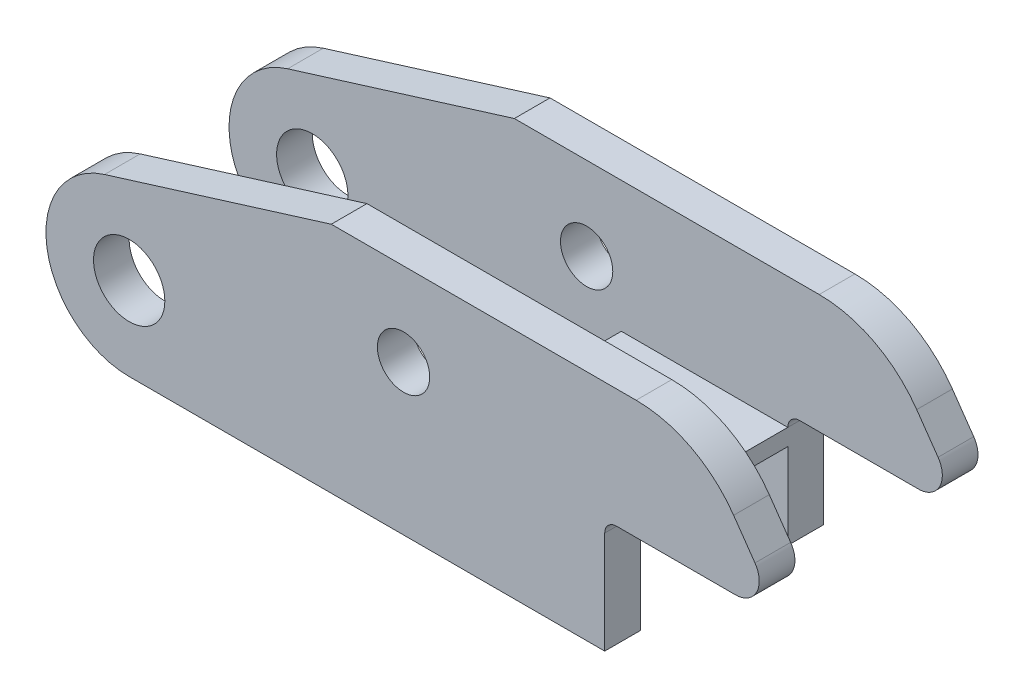
from build123d import *

# Parameters (mm, degrees)
EXTRUDE_START          = 700
SKETCH_1_R             = 15
EXTRUDE_1_DEPTH        = 15
PATTERN_LINEAR_1_COUNT = 2
PATTERN_LINEAR_1_PITCH = 77
SKETCH_2_W             = 62
SKETCH_2_H             = 7
EXTRUDE_2_DEPTH        = 70
SKETCH_3_R             = 11
CUT_EXTRUDE_2_DEPTH    = 105
FILLET_1_R             = 5


with BuildPart() as part:
    # 草图1 → 凸台-拉伸1 (new body)
    with BuildSketch(Plane.XY.offset(-2290.827909759).offset(EXTRUDE_START)):
        with BuildLine():
            Line((4, 81), (-196, 81))
            ThreePointArc((-196, 81), (-230.605231181, 110.758056189), (-206.365638709, 149.429830005))
            Line((-206.365638709, 149.429830005), (-111, 179))
            Line((-111, 179), (17.209362926, 179))
            ThreePointArc((17.209362926, 179), (40.340952707, 173.32752592), (58.22400875, 157.597182169))
            Line((58.22400875, 157.597182169), (67.202929165, 144.719436434))
            ThreePointArc((67.202929165, 144.719436434), (67.865505184, 134.373682044), (59, 129))
            Line((59, 129), (4, 129))
            Line((4, 129), (4, 81))
        make_face()
        with Locations((-196, 116)):
            Circle(SKETCH_1_R, mode=Mode.SUBTRACT)
    extrude(amount=EXTRUDE_1_DEPTH)


with BuildPart() as pattern_linear_1_1:
    # 阵列(线性)1: pattern copy
    add(part.part.moved(Location(Vector(0, 0, 1) * (1 * PATTERN_LINEAR_1_PITCH))))


with BuildPart() as part_1:
    add(part.part)

    add(pattern_linear_1_1.part)  # 凸台-拉伸2 merges 阵列(线性)1_1
    # 草图2 → 凸台-拉伸2 (add)
    with BuildSketch(Plane.ZY.offset(-4)):
        with Locations((-1544.827909759, 120.5)):
            Rectangle(SKETCH_2_W, SKETCH_2_H)
    extrude(amount=EXTRUDE_2_DEPTH)

    # 草图3 → 切除-拉伸2 (cut, symmetric)
    with BuildSketch(Plane(origin=(0, 0, -1513.827909759), x_dir=(-1, 0, 0), z_dir=(0, 0, -1))):
        with Locations(Location((80.605231181, 144, 0), (0, 0, 180))):
            Circle(SKETCH_3_R)
    extrude(amount=CUT_EXTRUDE_2_DEPTH, both=True, mode=Mode.SUBTRACT)

    # 圆角1
    fillet_1_edges = [part_1.edges().sort_by_distance(p)[0] for p in [
        (4, 129, -1583.327909759),
        (4, 129, -1506.327909759),
    ]]
    fillet(fillet_1_edges, radius=FILLET_1_R)


solid = part_1.part
